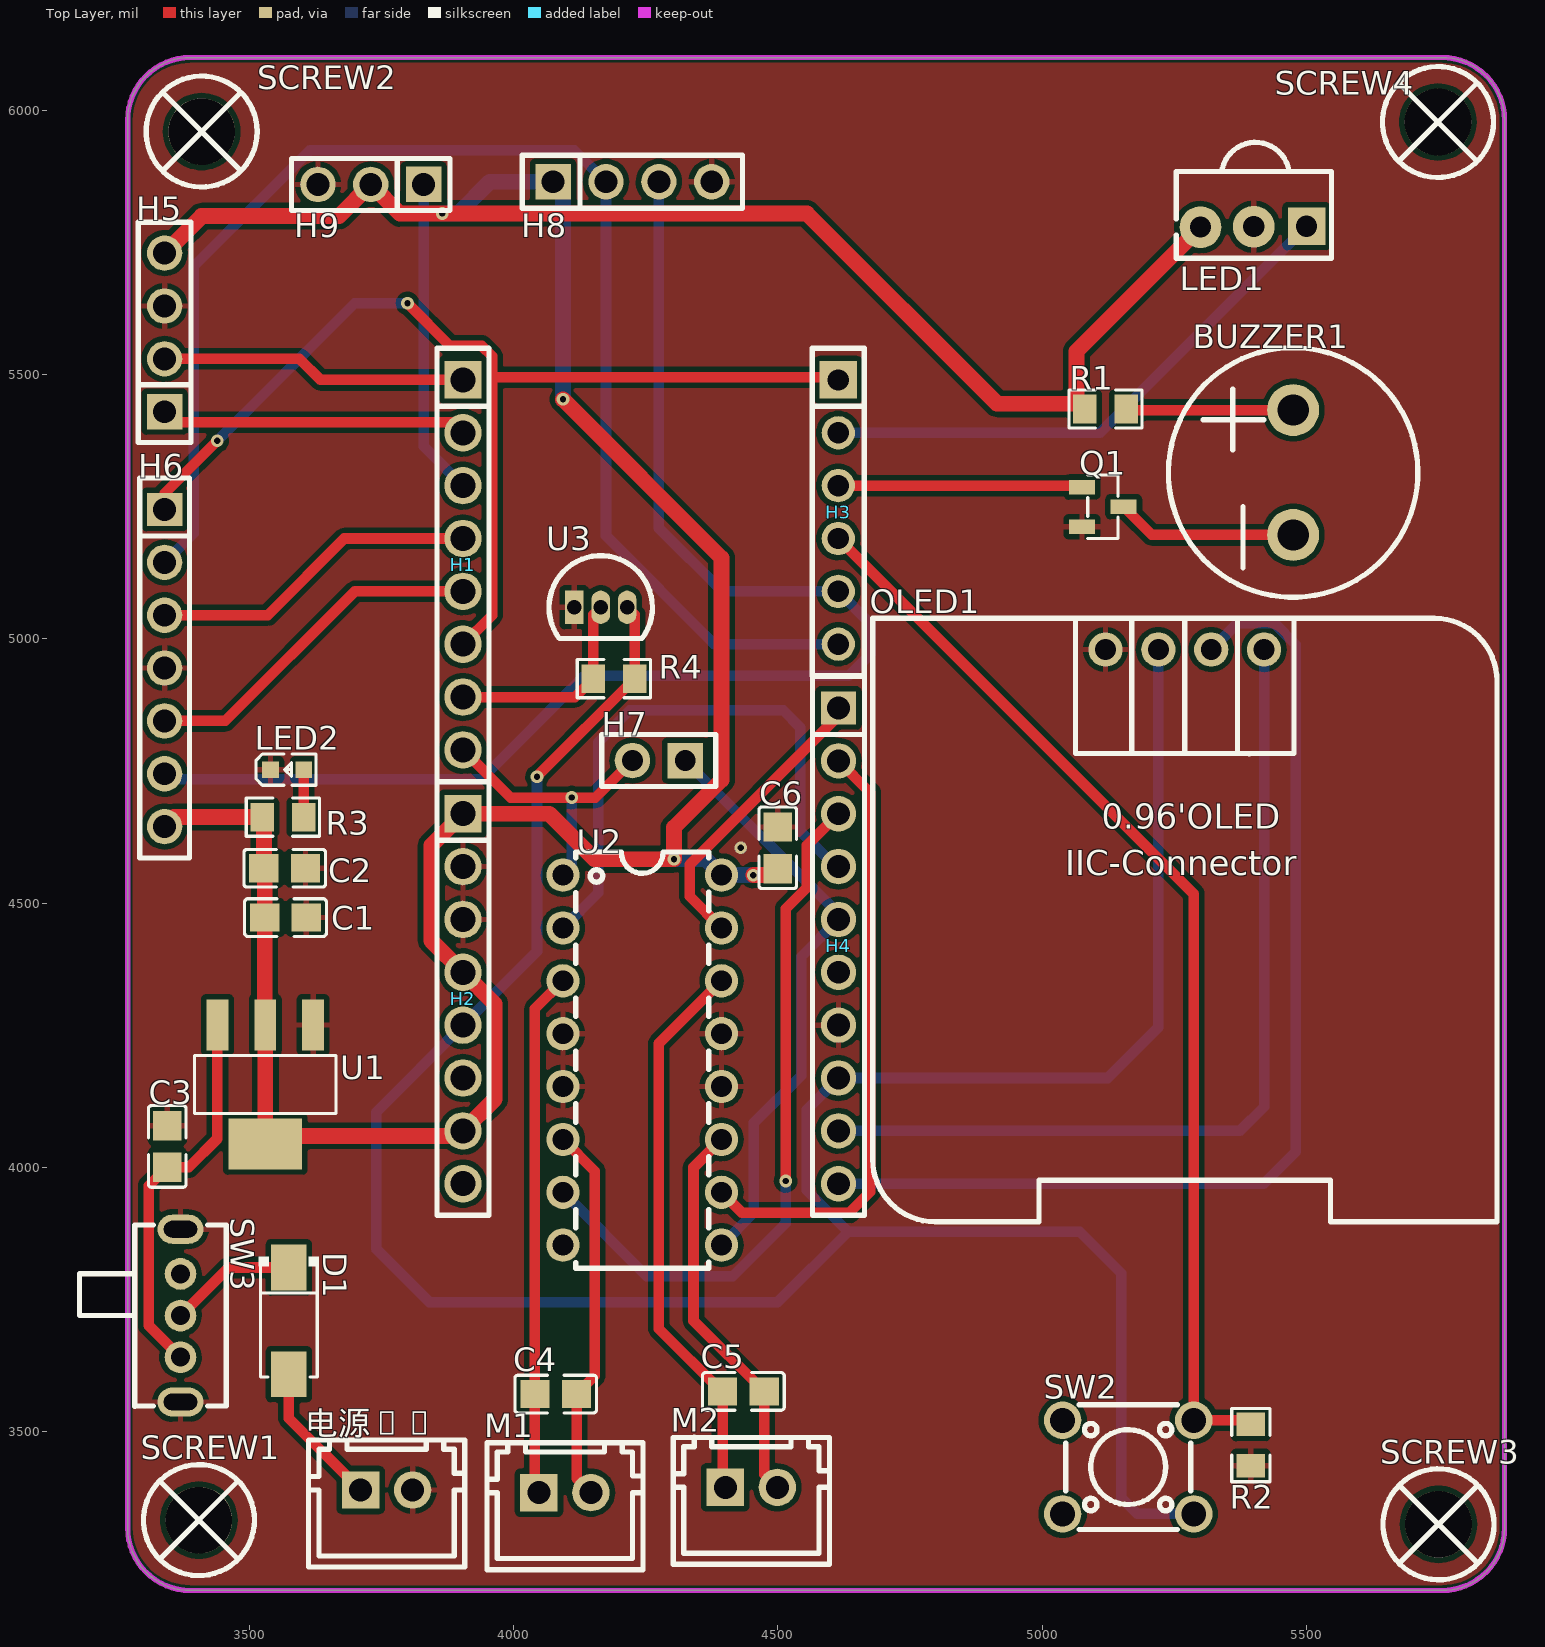
[diagram p0: Top Layer view]
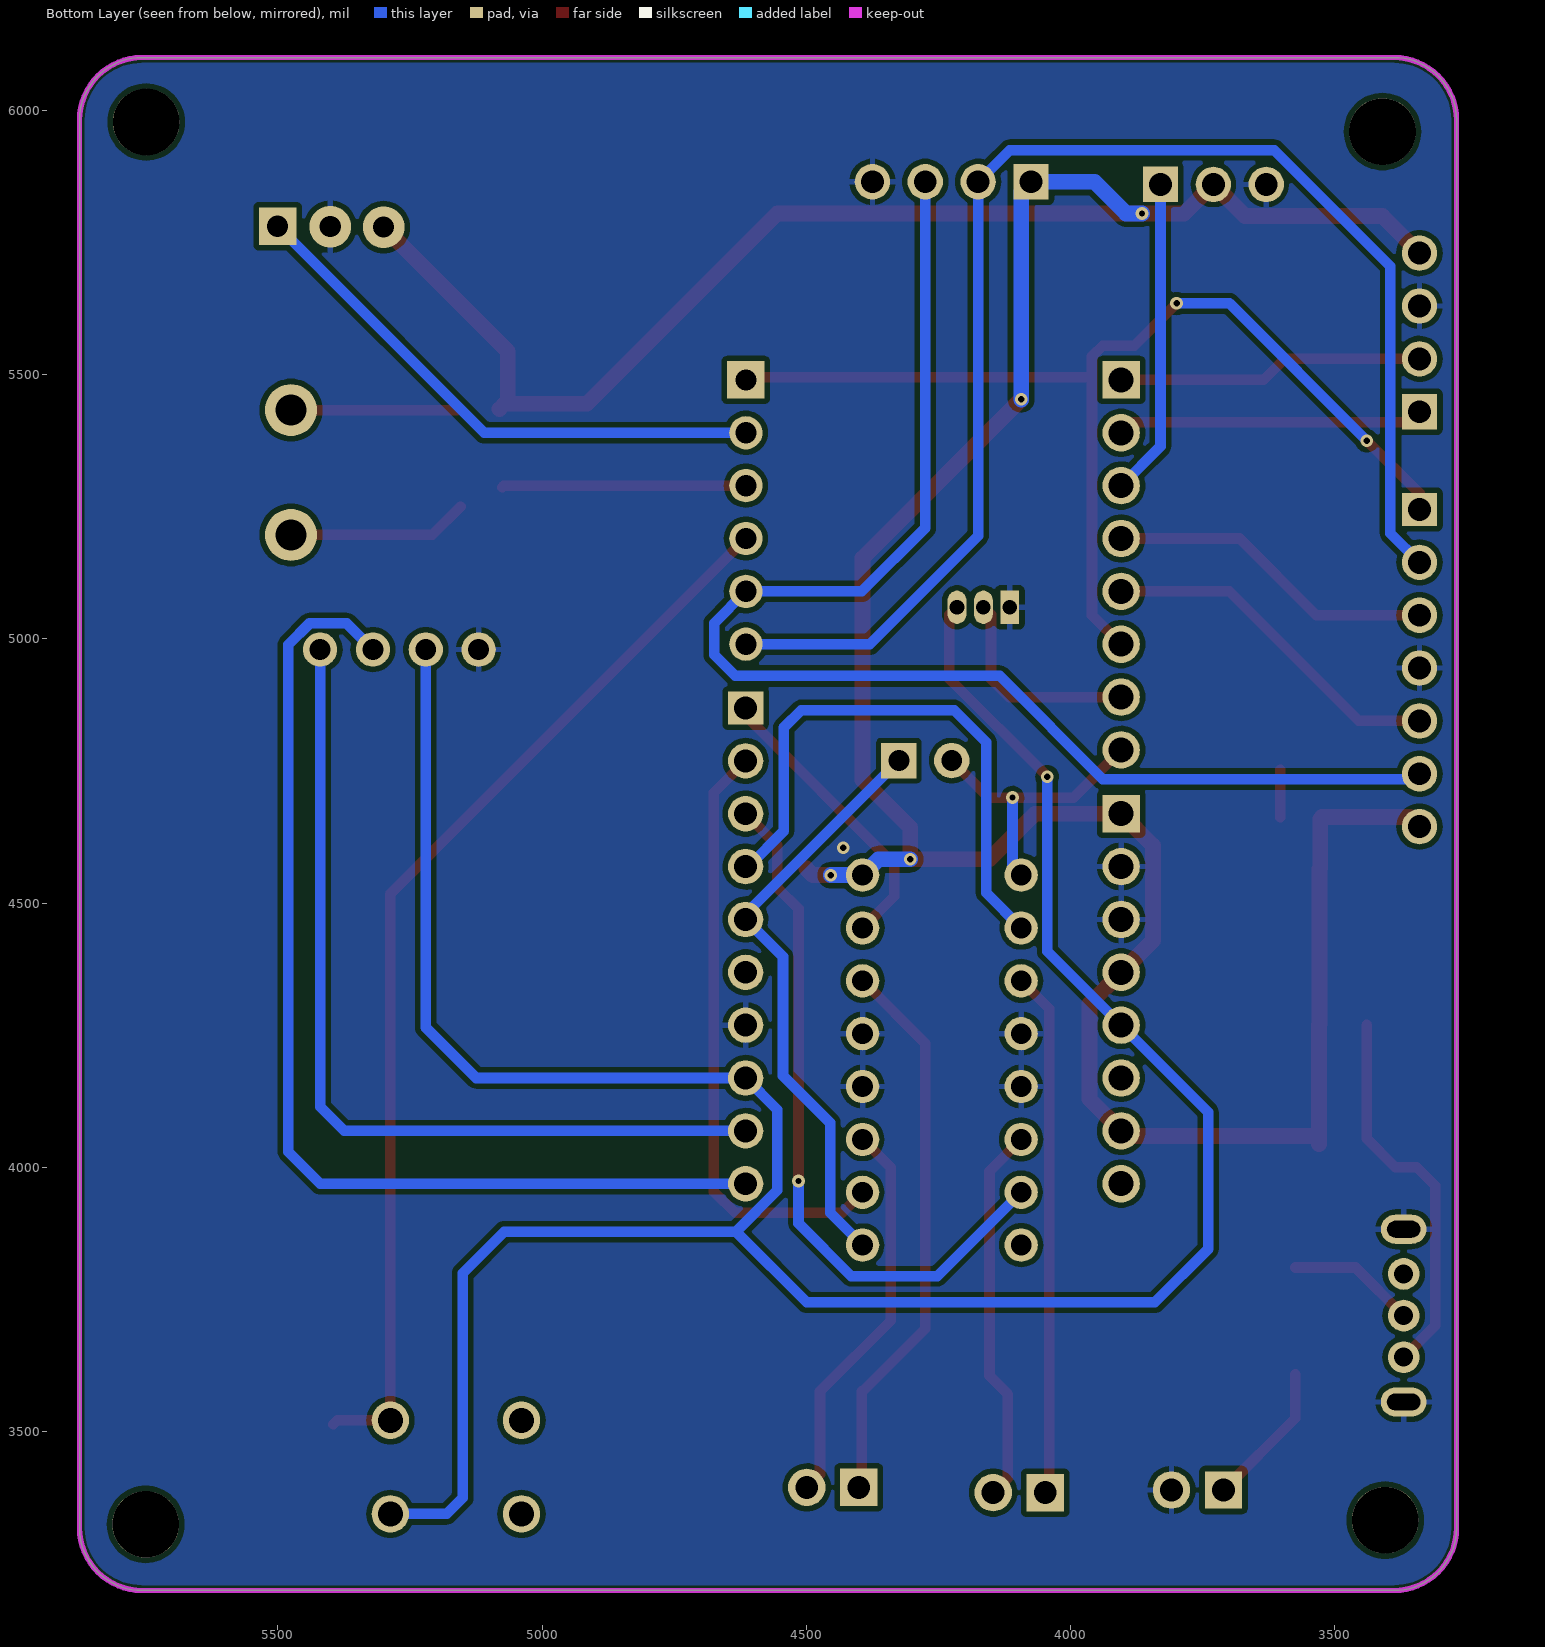
[diagram p1: Bottom Layer view, seen from below]
# Altium PCB MISC61257.pcbdoc
Units mil, origin at the board's own origin, x right, y up, seen from the top; angles counter-clockwise.
Board outline 2605 x 2900 mil, 2 copper layers (Top Layer, Bottom Layer), stack 62.206 mil thick; 37 components, 37 nets, 130 pads, 10 vias.

## Layer stack, top to bottom
Top Solder Mask Layer: solder mask 0.394, Dk 3.3
Top Layer: signal copper 1.379
Dielectric1: surface 59.449, FR4, Dk 4.5
Bottom Layer: signal copper 1.378
Bottom Solder Mask Layer: solder mask 0.394, Dk 3.3

## Board outline
3388.11,6100 ccw(c3388.11,5981.89) 3270,5981.89 3270,3318.11 ccw(c3388.11,3318.11) 3388.11,3200 5756.89,3200 ccw(c5756.89,3318.11) 5875,3318.11 5875,5981.89 ccw(c5756.89,5981.89) 5756.89,6100

## Design rules (kind name [scope] priority, off if disabled: settings)
BoardOutlineClearance copperThickness2oz_1 [All] p2 off: genericclearance=8 ignorepadtopadclearanceinfootprint=FALSE except(0: Arc-SplitContinuation Track-SplitContinuation SMDPad-SplitContinuation THPad-SplitContinuation Via-SplitContinuation Fill-SplitContinuation Region-SplitContinuation Poly-SplitContinuation Text-SplitContinuation Hole-SplitContinuation; 6: Arc-CutoutEdge Track-CutoutEdge SMDPad-CutoutEdge THPad-CutoutEdge Via-CutoutEdge Text-CutoutEdge; 6.9: Hole-OutlineEdge Hole-CutoutEdge; 10: Poly-OutlineEdge Poly-CutoutEdge; 11.8: Arc-OutlineEdge Track-OutlineEdge SMDPad-OutlineEdge THPad-OutlineEdge Via-OutlineEdge Fill-OutlineEdge Region-OutlineEdge Text-OutlineEdge Fill-CutoutEdge Region-CutoutEdge)
BoardOutlineClearance Plane_innerPlane_1 [All] p4 off: genericclearance=4 ignorepadtopadclearanceinfootprint=FALSE except(0: Arc-SplitContinuation Track-SplitContinuation SMDPad-SplitContinuation THPad-SplitContinuation Via-SplitContinuation Fill-SplitContinuation Region-SplitContinuation Poly-SplitContinuation Text-SplitContinuation Hole-SplitContinuation; 6: Arc-CutoutEdge Track-CutoutEdge SMDPad-CutoutEdge THPad-CutoutEdge Via-CutoutEdge Text-CutoutEdge; 6.9: Hole-OutlineEdge Hole-CutoutEdge; 10: Poly-OutlineEdge Poly-CutoutEdge; 11.8: Arc-OutlineEdge Track-OutlineEdge SMDPad-OutlineEdge THPad-OutlineEdge Via-OutlineEdge Fill-OutlineEdge Region-OutlineEdge Text-OutlineEdge Fill-CutoutEdge Region-CutoutEdge)
BoardOutlineClearance Copper_copperRegion_1 [All] p6 off: genericclearance=4 ignorepadtopadclearanceinfootprint=FALSE except(0: Arc-SplitContinuation Track-SplitContinuation SMDPad-SplitContinuation THPad-SplitContinuation Via-SplitContinuation Fill-SplitContinuation Region-SplitContinuation Poly-SplitContinuation Text-SplitContinuation Hole-SplitContinuation; 6: Arc-CutoutEdge Track-CutoutEdge SMDPad-CutoutEdge THPad-CutoutEdge Via-CutoutEdge Text-CutoutEdge; 6.9: Hole-OutlineEdge Hole-CutoutEdge; 10: Poly-OutlineEdge Poly-CutoutEdge; 11.8: Arc-OutlineEdge Track-OutlineEdge SMDPad-OutlineEdge THPad-OutlineEdge Via-OutlineEdge Fill-OutlineEdge Region-OutlineEdge Text-OutlineEdge Fill-CutoutEdge Region-CutoutEdge)
BoardOutlineClearance copperThickness1oz_1 [All] p8: genericclearance=4 ignorepadtopadclearanceinfootprint=FALSE except(0: Arc-SplitContinuation Track-SplitContinuation SMDPad-SplitContinuation THPad-SplitContinuation Via-SplitContinuation Fill-SplitContinuation Region-SplitContinuation Poly-SplitContinuation Text-SplitContinuation Hole-SplitContinuation; 6: Arc-CutoutEdge Track-CutoutEdge SMDPad-CutoutEdge THPad-CutoutEdge Via-CutoutEdge Text-CutoutEdge; 6.9: Hole-OutlineEdge Hole-CutoutEdge; 10: Poly-OutlineEdge Poly-CutoutEdge; 11.8: Arc-OutlineEdge Track-OutlineEdge SMDPad-OutlineEdge THPad-OutlineEdge Via-OutlineEdge Fill-OutlineEdge Region-OutlineEdge Text-OutlineEdge Fill-CutoutEdge Region-CutoutEdge)
Clearance copperThickness2oz [All] p1 off: gap=8 ignorepadtopadclearanceinfootprint=FALSE except(6: SMDPad-Track SMDPad-SMDPad THPad-Track SMDPad-THPad THPad-THPad Track-Via SMDPad-Via THPad-Via Via-Via Fill-SMDPad Region-SMDPad Fill-THPad Region-THPad Fill-Via Region-Via Fill-Fill Fill-Region Region-Region Arc-Track Arc-SMDPad Arc-THPad Arc-Via Fill-Arc Region-Arc Arc-Arc Text-Track SMDPad-Text Text-THPad Text-Via Fill-Text Region-Text Arc-Text Text-Text; 6.9: Hole-Track Hole-SMDPad Hole-THPad Hole-Via Fill-Hole Region-Hole Hole-Arc Hole-Text; 10: Poly-Track Poly-SMDPad Poly-THPad Poly-Via Poly-Fill Poly-Region Poly-Poly Poly-Arc Poly-Text Poly-Hole; 11.8: Fill-Track Region-Track)
Clearance Plane_innerPlane [All] p3 off: gap=4 ignorepadtopadclearanceinfootprint=FALSE except(6: SMDPad-Track SMDPad-SMDPad THPad-Track SMDPad-THPad THPad-THPad Track-Via SMDPad-Via THPad-Via Via-Via Fill-SMDPad Region-SMDPad Fill-THPad Region-THPad Fill-Via Region-Via Fill-Fill Fill-Region Region-Region Arc-Track Arc-SMDPad Arc-THPad Arc-Via Fill-Arc Region-Arc Arc-Arc Text-Track SMDPad-Text Text-THPad Text-Via Fill-Text Region-Text Arc-Text Text-Text; 6.9: Hole-Track Hole-SMDPad Hole-THPad Hole-Via Fill-Hole Region-Hole Hole-Arc Hole-Text; 10: Poly-Track Poly-SMDPad Poly-THPad Poly-Via Poly-Fill Poly-Region Poly-Poly Poly-Arc Poly-Text Poly-Hole; 11.8: Fill-Track Region-Track)
Clearance Copper_copperRegion [All] p5 off: gap=4 ignorepadtopadclearanceinfootprint=FALSE except(6: SMDPad-Track SMDPad-SMDPad THPad-Track SMDPad-THPad THPad-THPad Track-Via SMDPad-Via THPad-Via Via-Via Fill-SMDPad Region-SMDPad Fill-THPad Region-THPad Fill-Via Region-Via Fill-Fill Fill-Region Region-Region Arc-Track Arc-SMDPad Arc-THPad Arc-Via Fill-Arc Region-Arc Arc-Arc Text-Track SMDPad-Text Text-THPad Text-Via Fill-Text Region-Text Arc-Text Text-Text; 6.9: Hole-Track Hole-SMDPad Hole-THPad Hole-Via Fill-Hole Region-Hole Hole-Arc Hole-Text; 10: Poly-Track Poly-SMDPad Poly-THPad Poly-Via Poly-Fill Poly-Region Poly-Poly Poly-Arc Poly-Text Poly-Hole; 11.8: Fill-Track Region-Track)
Clearance copperThickness1oz [All] p7: gap=4 ignorepadtopadclearanceinfootprint=FALSE except(6: SMDPad-Track SMDPad-SMDPad THPad-Track SMDPad-THPad THPad-THPad Track-Via SMDPad-Via THPad-Via Via-Via Fill-SMDPad Region-SMDPad Fill-THPad Region-THPad Fill-Via Region-Via Fill-Fill Fill-Region Region-Region Arc-Track Arc-SMDPad Arc-THPad Arc-Via Fill-Arc Region-Arc Arc-Arc Text-Track SMDPad-Text Text-THPad Text-Via Fill-Text Region-Text Arc-Text Text-Text; 6.9: Hole-Track Hole-SMDPad Hole-THPad Hole-Via Fill-Hole Region-Hole Hole-Arc Hole-Text; 10: Poly-Track Poly-SMDPad Poly-THPad Poly-Via Poly-Fill Poly-Region Poly-Poly Poly-Arc Poly-Text Poly-Hole; 11.8: Fill-Track Region-Track)
DiffPairsRouting differentialPair [All] p1: maxlimit=6 minlimit=6 mostfreqgap=6 toplayer_minwidth=5 toplayer_prefwidth=10 toplayer_maxwidth=100 toplayer_mingap=6 toplayer_prefgap=6 toplayer_maxgap=6 bottomlayer_minwidth=5 bottomlayer_prefwidth=10 bottomlayer_maxwidth=100 bottomlayer_mingap=6 bottomlayer_prefgap=6 bottomlayer_maxgap=6 maxuncoupledlength=10
HoleToHoleClearance otherClearance [All] p1: gap=11.8 allowstackedmicrovias=TRUE
Length netLength [All] p1: minlimit=0 maxlimit=0
PasteMaskExpansion pasteMaskExpansion [All] p1: expansion=0
PlaneConnect innerPlane [All] p1: planeconnectstyle=Relief reliefexpansion=20 reliefentries=4 reliefconductorwidth=10 reliefairgap=10
PolygonConnect copperRegion [All] p1: connectstyle=Relief reliefconductorwidth=10 reliefentries=4 polygonreliefangle="90 Angle" airgapwidth=10 via.connectstyle=Relief via.reliefconductorwidth=10 via.reliefentries=4 via.polygonreliefangle="90 Angle" via.airgapwidth=10
RoutingVias viaSize [All] p1: holewidth=12 width=24 viastyle="Through Hole" minholewidth=11.8 minwidth=19.7 maxholewidth=248 maxwidth=393.7
SolderMaskExpansion solderMaskExpansion [IsVia] p1: expansion=-1000 istentingtop=TRUE
SolderMaskExpansion solderMaskExpansion [All] p2: expansion=2 istentingtop=FALSE
Width copperThickness2oz_2 [All] p1 off: maxlimit=100 minlimit=8 preferedwidth=10
Width copperThickness1oz_2 [All] p2: maxlimit=100 minlimit=20 preferedwidth=30

## Components (designator, comment, footprint, x,y, rotation, side; value= is the part's Value field where it differs from the comment)
BUZZER1 "buzzer" BUZ-TH_BD12.0-P6.00-D0.9-RD 5475,5315 r90 top
C1 "10uF" C0805 3568.66,4472.94 r180 top
C2 "100nF" C0805 3567.19,4566.27 r180 top
C3 "10uF" C0805 3345,4040 r270 top
C4 "100nF" C0805 4079.91,3571.55 r0 top
C5 "100nF" C0805 4434.87,3576.55 r0 top
C6 "100nF" C0805 4500,4605 r270 top
D1 "SS14" SMA_L4.2-W2.6-LS5.3-RD 3575,3710 r270 top
H1 "" HDR-TH_8P-P2.54-V-F-1 3904.43,5140.14 r270 top
H2 "" HDR-TH_8P-P2.54-V-F-1 3904.43,4319.43 r270 top
H3 "" HDR-TH_6P-P2.54-V-F 4614.43,5240.14 r270 top
H4 "" HDR-TH_10P-P2.54-V-F 4614.86,4419.43 r270 top
H5 "" HDR-TH_4P-P2.54-V-F 3340,5580 r90 top
H6 "" HDR-TH_7P-P2.54-V-F 3340,4945 r270 top
H7 "" HDR-TH_2P-P2.54-V-F 4275,4770 r180 top
H8 "" HDR-TH_4P-P2.54-V-F 4225,5865 r0 top
H9 "" HDR-TH_3P-P2.54-V-M 3730,5860 r180 top
LED1 "TSDP34138" SENSOR-TH_TSDP34138 5400,5780 r180 top
LED2 "" LED_0603 3573.66,4752.94 r0 top
M1 "HX25003-2A" CONN-TH_2P-P2.50_HX25003-2A 4097.34,3385 r0 top
M2 "HX25003-2A" CONN-TH_2P-P2.50_HX25003-2A 4450,3395 r0 top
OLED1 "" 0.96OLED_4P 5270,4980 r0 top
Q1 "SS8050" SOT-23-3_L2.9-W1.3-P1.90-LS2.4-BR 5115,5250 r180 top
R1 "200Ω" R0805 5120,5435 r180 top
R2 "4.7K" R0805 5395,3475 r90 top
R3 "4.7K" R0805 3563.66,4662.94 r180 top
R4 "4.7KΩ" R0805 4190,4925 r0 top
SCREW1 "" M3螺丝 3404.9,3333.05 r0 top
SCREW2 "" M3螺丝 3410,5960 r0 top
SCREW3 "" M3螺丝 5750,3325 r0 top
SCREW4 "" M3螺丝 5748.95,5978.05 r0 top
SW2 "TS1702-CZ65HBS" SW-TH_4P-L6.0-W6.0-P4.50-LS6.3 5162.93,3433.35 r0 top
SW3 "SK12D07VG4" SW-TH_SK12D07VG4 3370,3720 r270 top
U1 "AMS1117-5.0" SOT-223_L6.5-W3.5-P2.30-LS7.0-BR 3530.46,4157.23 r90 top
U2 "L293D" DIP-16_L20.0-W6.4-P2.54-LS7.6-BL 4243.58,4203.29 r270 top
U3 "DS18B20+" TO-92-3_L4.9-W3.7-P1.27-L 4165,5060 r0 top
电源IN "HX25003-2A" CONN-TH_2P-P2.50_HX25003-2A 3760,3390 r0 top

## Footprints (in the part's own frame and the unit in brackets; to place one, negate y for a bottom-side part, rotate by r counter-clockwise, add the part's x,y. Pads: shape width x height; smd on the part's side, far side on the other; paste and mask are expansions set on the pad)
0.96OLED_4P [mm]
  round 1.65 hole 1 copper offset 0,0: 1(-3.81,-0.001) 2(-1.27,0.002) 3(1.27,0.002) 4(3.81,0.002)
  silkscreen extent -15,-27.5 15,1.5
BUZ-TH_BD12.0-P6.00-D0.9-RD [mm]
  round 2.5 hole 1.5 paste+0 mask+0.05: 1(-3,0) 2(3,0)
  silkscreen extent -5.99,-5.99 5.99,5.99
C0805 [mm]
  rect 1.41x1.35 smd paste-100 mask+0.051: 1(-1,0) 2(1,0)
  silkscreen extent -1.96,-0.9 1.96,0.9
CONN-TH_2P-P2.50_HX25003-2A [mm]
  rect 1.8x1.8 hole 1.1 paste+0 mask+0.05: 1(-1.25,0)
  round 1.8 hole 1.1 paste+0 mask+0.05: 2(1.25,0)
  silkscreen extent -3.75,-3.7 3.75,2.41
DIP-16_L20.0-W6.4-P2.54-LS7.6-BL [mm]
  round 1.6 hole 1: 1(-8.89,-3.81) 2(-6.35,-3.81) 3(-3.81,-3.81) 4(-1.27,-3.81) 5(1.27,-3.81) 6(3.81,-3.81) 7(6.35,-3.81) 8(8.89,-3.81) 9(8.89,3.81) 10(6.35,3.81) 11(3.81,3.81) 12(1.27,3.81) 13(-1.27,3.81) 14(-3.81,3.81) 15(-6.35,3.81) 16(-8.89,3.81)
  silkscreen extent -10,-3.2 10,3.2
HDR-TH_2P-P2.54-V-F [mm]
  rect 1.7x1.7 hole 1: 1(-1.27,0)
  round 1.7 hole 1: 2(1.27,0)
  silkscreen extent -2.74,-1.25 2.74,1.25
HDR-TH_3P-P2.54-V-M [mm]
  rect 1.7x1.7 hole 1.1: 1(-2.54,0)
  round 1.7 hole 1.1: 2(0,0) 3(2.54,0)
  silkscreen extent -3.81,-1.25 3.81,1.25
HDR-TH_4P-P2.54-V-F [mm]
  rect 1.7x1.7 hole 1.1: 1(-3.81,0)
  round 1.7 hole 1.1: 2(-1.27,0) 3(1.27,0) 4(3.81,0)
  silkscreen extent -5.29,-1.27 5.29,1.27
HDR-TH_6P-P2.54-V-F [mm]
  rect 1.8x1.8 hole 1.02: 1(-6.35,0)
  round 1.6 hole 1.02: 2(-3.81,0) 3(-1.27,0) 4(1.27,0) 5(3.81,0) 6(6.35,0)
  silkscreen extent -7.87,-1.25 7.87,1.25
HDR-TH_7P-P2.54-V-F [mm]
  rect 1.575x1.7 hole 1.1: 1(-7.62,0)
  round 1.7 hole 1.1: 2(-5.08,0) 3(-2.54,0) 4(0,0) 5(2.54,0) 6(5.08,0) 7(7.62,0)
  silkscreen extent -9.13,-1.2 9.13,1.2
HDR-TH_8P-P2.54-V-F-1 [mm]
  rect 1.8x1.8 hole 1.2: 1(-8.89,0)
  round 1.8 hole 1.2: 2(-6.35,0) 3(-3.81,0) 4(-1.27,0) 5(1.27,0) 6(3.81,0) 7(6.35,0) 8(8.89,0)
  silkscreen extent -10.41,-1.25 10.41,1.25
HDR-TH_10P-P2.54-V-F [mm]
  rect 1.575x1.7 hole 1.1: 1(-11.43,0)
  round 1.7 hole 1.1: 2(-8.89,0) 3(-6.35,0) 4(-3.81,0) 5(-1.27,0) 6(1.27,0) 7(3.81,0) 8(6.35,0) 9(8.89,0) 10(11.43,0)
  silkscreen extent -12.95,-1.25 12.95,1.25
LED_0603 [mil]
  rect 31.5x31.5 smd paste+0 mask+2: 1(-33.5,-0.4) 2(29.5,-0.2)
  silkscreen extent -61,-30 53,30
M3螺丝 [mil]
  round 126 hole 126 paste+0 mask+4: 1(0,0)
  silkscreen extent -105,-105 105,105
R0805 [mm]
  rect 1.133x1.377 smd paste-100 mask+0.051: 1(-1,0) 2(1,0)
  silkscreen extent -1.76,-0.92 1.76,0.92
SENSOR-TH_TSDP34138 [mil]
  rect 71x71 hole 40: 1(-100.3,-0.81)
  round 79 hole 40: 2(-0.6,-0.09) 3(100.3,0.81)
  silkscreen extent -148,-160 146,60
SMA_L4.2-W2.6-LS5.3-RD [mm]
  rect 2.2x1.7 smd: 1(-2.565,0) 2(2.565,0)
  silkscreen extent -3.08,-1.44 2.7,1.44
SOT-23-3_L2.9-W1.3-P1.90-LS2.4-BR [mm]
  rect 1.25x0.7 smd: 1(1,-0.95) 2(1,0.95) 3(-1,0)
  silkscreen extent -0.73,-1.53 0.73,1.53
SOT-223_L6.5-W3.5-P2.30-LS7.0-BR [mm]
  rect 2.465x1.05 smd: 1(2.857,-2.3) 2(2.857,0) 3(2.857,2.3)
  rect 2.465x3.54 smd: 4(-2.857,0)
  silkscreen extent -1.4,-3.4 1.4,3.4
SW-TH_4P-L6.0-W6.0-P4.50-LS6.3 [mm]
  round 1.8 hole 1.2: 1(-3.15,2.25) 2(3.15,2.25) 3(-3.15,-2.25) 4(3.15,-2.25)
  silkscreen extent -3,-3 3,3
SW-TH_SK12D07VG4 [mil]
  round 60 hole 36 paste+0 mask+1.97: 1(-78.74,0) 2(0,0) 3(78.74,0)
  oval 55.12x86.61 hole 31.5 slot 62.99 at 90 deg paste+0 mask+1.97: 4(163.38,0) 5(-163.39,0)
  silkscreen extent -171,-191 171,87
TO-92-3_L4.9-W3.7-P1.27-L [mm]
  rect 0.9x1.6 hole 0.7: 1(-1.27,0)
  oval 0.9x1.6 hole 0.7: 2(0,0) 3(1.27,0)
  silkscreen extent -2.48,-1.5 2.48,2.48

## Via types
v1: diameter 24, hole 12, Top Layer to Bottom Layer, 6 vias
v2: diameter 24.02, hole 12, Top Layer to Bottom Layer, 4 vias

## Nets (pads, with @x,y where several pads share a name; then routed paths per layer and width w, separated by ;. In a path a pad name is that pad's centre, name@x,y a point inside that pad or via, vN(x,y) a via of type N, cw(c..) or ccw(c..) an arc to the next point about the centre after c; other vN are vias at no path point)
3.3V: H2.5 H4.8 OLED1.2 R4.2 SW2.4 U3.3 | length 5244.7
  Top Layer w20: v2(4044.43,4739.43) 4044.43,4740.06 R4.2 4229.37,5045.63 U3.3
  Bottom Layer w20: v2(4044.43,4739.43) 4044.43,4409.43 H2.5 3740,4105 3740,3845.99 3840.99,3745 4499.49,3745 4633.1,3878.61 ; OLED1.2@5220,4980.05 5220,4265 5124.43,4169.43 H4.8 4554.86,4109.43 4554.86,3956.85 4633.1,3878.61 ; SW2.4 5180.23,3344.77 5150,3375 5150,3800 5071.39,3878.61 4633.1,3878.61
$1N1420: BUZZER1.2 R1.1 | length 316.4
  Top Layer w20: R1.1 5161.26,5433.11 BUZZER1.2
$1N1485: BUZZER1.1 Q1.3 | length 342.6
  Top Layer w20: Q1.3 5207.48,5196.89 BUZZER1.1
$1N2734: LED2.2 R3.1 | length 89.7
  Top Layer w20: R3.1@3603.16,4663.07 LED2.2
$1N2901: C3.2 SW3.3 U1.3 | length 730.9
  Top Layer w20: SW3.3 3310,3701.26 3310,3965.63 C3.2 3385.63,4000.63 3439.91,4054.91 U1.3
$1N3240: D1.1 SW3.2 | length 242.7
  Top Layer w20: SW3.2 3461,3811 D1.1
$1N3307: D1.2 电源IN.1 | length 275.2
  Top Layer w20: D1.2 3575,3525.79 电源IN.1
$1N4775: C4.1 M1.1 U2.3 | length 993.4
  Top Layer w20: M1.1 4040.53,3392.59 C4.1 4040.53,4300.25 U2.3
$1N4781: C4.2 M1.2 U2.6 | length 718.6
  Top Layer w20: U2.6 4153.58,3993.29 4153.58,3605.85 C4.2 4119.27,3412.27 M1.2@4146.55,3385
$1N4892: C5.1 M2.1 U2.14 | length 1060.7
  Top Layer w20: U2.14 4275,4234.71 4275,3695 4393.45,3576.55 C5.1 4395.5,3400.29 M2.1
$1N4896: C5.2 M2.2 U2.11 | length 746.1
  Top Layer w20: U2.11 4340.5,4000.21 4340.5,3710.13 4474.08,3576.55 C5.2 4474.24,3419.97 M2.2
+5V: C1.2 C2.2 C6.2 H2.1 H2.4 H2.7 H5.4 H6.7 H8.1 H9.2 LED1.3 R1.2 R3.2 U1.2 U1.4 U2.16 | length 6626.4
  Top Layer w30: H6.7 3357.94,4662.94 R3.2 3527.82,4659.41 C2.2 3529.29,4564.81 C1.2 3529.29,4270.9 U1.2 U1.4@3530.46,4059.73 ; H5.4 3410,5800 3670,5800 H9.2 3785,5805 v1(3865,5805) 4555,5805 4915,5445 R1.2@5065,5445 ; U1.4 U1.4@3530.46,4059.73 ; v1(4093.58,5453.29) 4393.58,5153.29 4393.58,4733.29 4303.58,4643.29 v1(4303.58,4583.29) 4153.58,4583.29 4067.44,4669.43 H2.1 3844.43,4609.43 3844.43,4429.43 H2.4 3964.43,4309.43 3964.43,4129.43 H2.7 3894.73,4059.73 U1.4@3530.46,4059.73 ; v1(4453.58,4553.29) 4487.66,4553.29 C6.2 ; R1.2 5070.63,5445 R1.2@5065,5445 ; LED1.3 5065,5544.49 R1.2@5065,5445
  Bottom Layer w30: v1(3865,5805) 3895,5805 3955,5865 H8.1 4093.58,5846.42 v1(4093.58,5453.29) ; v1(4303.58,4583.29) 4363.58,4583.29 U2.16 v1(4453.58,4553.29)
A0: H3.6 H6.2 H8.2 | length 2673
  Bottom Layer w20: H6.2 3395,5200 3395,5705 3615,5925 4115,5925 H8.2 4175,5195 4379.86,4990.14 H3.6
A1: H3.5 H6.6 H8.3 | length 2624.9
  Bottom Layer w20: H6.6 3350,4735 3939.29,4735 4134.43,4930.14 4634.43,4930.14 4674.43,4970.14 4674.43,5030.14 H3.5 4394.86,5090.14 4275,5210 H8.3
BEEP: H3.3 Q1.1 | length 462.3
  Top Layer w20: H3.3 5072.89,5290.14 Q1.1
D2: H1.3 H9.1 | length 600.7
  Bottom Layer w20: H9.1 3830,5364.57 H1.3
D3: H1.4 H6.3 | length 624.5
  Top Layer w20: H6.3 3535,5045 3680.14,5190.14 H1.4
D4: H1.5 H6.5 | length 666
  Top Layer w20: H6.5 3455,4845 3700.14,5090.14 H1.5
D5: H1.6 H3.1 H6.1 | length 2064.9
  Top Layer w20: H6.1 3340,5275.43 v2(3439.57,5375) ; v2(3799.57,5635) 3879.57,5555 3939.57,5555 3959.57,5535 3959.57,5495 ; H1.6 3959.57,5045.28 3959.57,5495 ; H3.1 4609.57,5495 3959.57,5495
  Bottom Layer w20: v2(3439.57,5375) 3699.57,5635 v2(3799.57,5635)
DQ: H1.7 R4.1 U3.2 | length 401.6
  Top Layer w20: H1.7 4115.77,4890.14 R4.1 4150.63,5045.63 U3.2
GND: C1.1 C2.1 C3.1 C6.1 H2.2 H2.3 H4.7 H5.3 H6.4 H8.4 H9.3 LED1.2 LED2.1 OLED1.1 Q1.2 R2.1 SW3.4 SW3.5 U1.1 U2.4 U2.5 U2.12 U2.13 U3.1 电源IN.2
  other v1: 4430,4605
INBAT: U2.8
INPUT1: H4.4 U2.2 | length 1096
  Bottom Layer w20: U2.2 4160,4519.71 4160,4805 4220,4865 4510,4865 4542.49,4832.51 4542.49,4636.81 4609.86,4569.43 H4.4
INPUT2: H4.3 U2.7 | length 1344.7
  Top Layer w20: v2(4514.86,3974.58) 4514.86,4489.43 4554.86,4529.43 4554.86,4609.43 H4.3
  Bottom Layer w20: U2.7 4252.29,3794.58 4414.86,3794.58 4514.86,3894.58 v2(4514.86,3974.58)
INPUT3: H4.2 U2.10 | length 1153.6
  Top Layer w20: U2.10 4432.29,3914.58 4634.86,3914.58 4674.86,3954.58 4674.86,4709.43 H4.2
INPUT4: H4.1 U2.15 | length 557.5
  Top Layer w20: U2.15 4333.58,4513.29 4333.58,4573.29 4614.86,4854.58 H4.1
KEY: H3.4 R2.2 SW2.2 | length 2058
  Top Layer w20: H3.4 5286.95,4517.62 SW2.2 5387.44,3521.93 R2.2
NRST: H2.6
PA5: H3.2 LED1.1 | length 1047.7
  Bottom Layer w20: H3.2 5109.63,5390.14 LED1.1
PA8: H1.8 H7.2 U2.1 | length 540.4
  Top Layer w20: H1.8 3994.57,4700 v1(4110,4700) 4155,4700 H7.2
  Bottom Layer w20: U2.1 4110,4569.71 v1(4110,4700)
PA9: H1.2 H5.1 | length 580.9
  Top Layer w20: H5.1 3360,5410 3884.57,5410 H1.2
PA10: H1.1 H5.2 | length 580.9
  Top Layer w20: H5.2 3595,5530 3634.86,5490.14 H1.1
PB10: H4.10 OLED1.3 | length 2046.7
  Bottom Layer w20: H4.10 5419.43,3969.43 5480,4030 5480,4989.43 5440,5029.43 5369.38,5029.43 OLED1.3@5320,4980.05
PB11: H4.9 OLED1.4 | length 1689.1
  Bottom Layer w20: H4.9 5374.43,4069.43 5420,4115 OLED1.4@5420,4980.05
PB14: H4.5 H7.1 U2.9 | length 1128.4
  Bottom Layer w20: H7.1 4614.86,4480.14 H4.5 4544.23,4398.8 4544.23,4173.8 4454.86,4084.43 4454.86,3914.58 U2.9
PB15: H4.6
VBAT: H2.8
pads on no net: SCREW1.1 SCREW2.1 SCREW3.1 SCREW4.1 SW2.1 SW2.3 SW3.1

## Polygon pours and split planes (outlines as drawn)
GND on Top Layer (solid, remove dead copper, pour order 0): 3000,6120 3000,3000 6280,3000 6280,6120
GND on Bottom Layer (solid, remove dead copper, pour order 2): 3090,6130 3090,3080 6165,3080 6165,6130

## Keep-outs
Board Outline Layer:
  the board outline again, w10